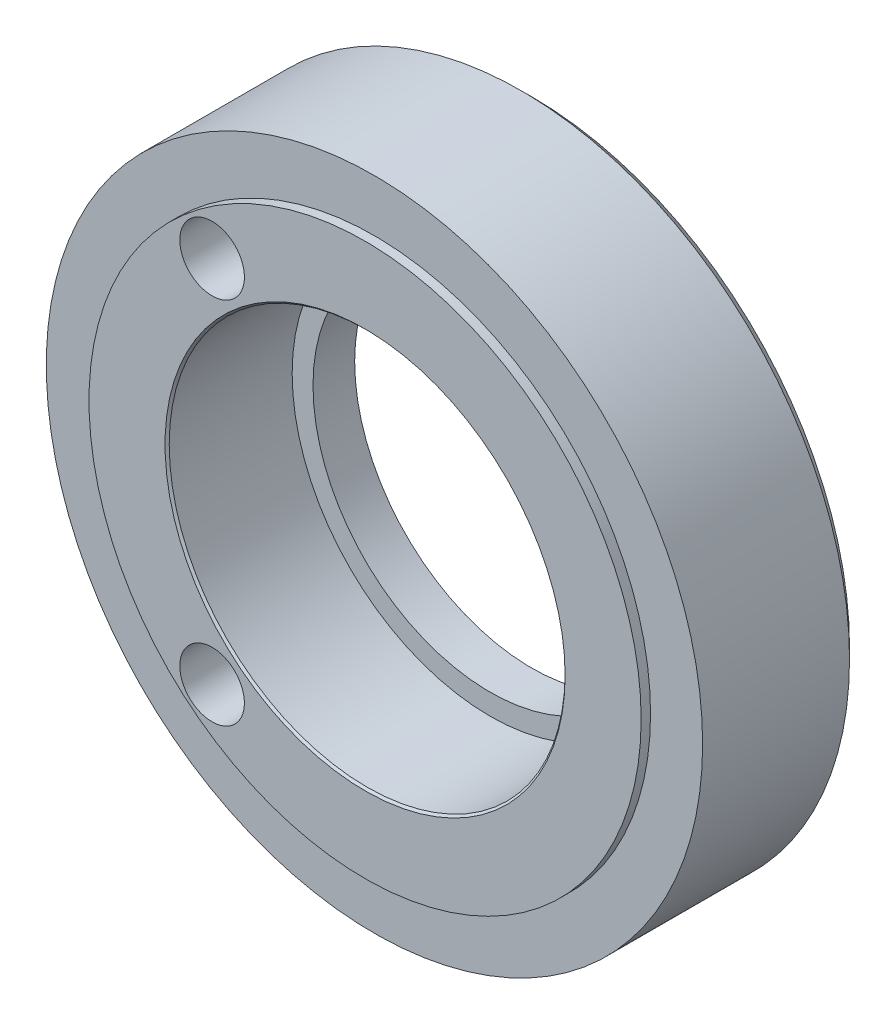
from build123d import *

# Parameters (mm, degrees)
SKETCH1_R                  = 15.75
SKETCH1_R_2                = 9.5
BOSS_EXTRUDE1_DEPTH        = 4
SKETCH3_R                  = 10.639095477
SKETCH3_R_2                = 8.5
BOSS_EXTRUDE2_DEPTH        = 2
F_3_1_3_1_DIAMETER_HOLE1_D = 3.1
SKETCH7_R                  = 18.245705154
SKETCH7_R_2                = 13.25
CUT_EXTRUDE1_DEPTH         = 0.45
CHAMFER1_SIZE              = 0.5
CHAMFER2_SIZE              = 0.1


with BuildPart() as part:
    # Sketch1 → Boss-Extrude1 (new, symmetric)
    with BuildSketch(Plane.XY):
        Circle(SKETCH1_R)
        Circle(SKETCH1_R_2, mode=Mode.SUBTRACT)
    extrude(amount=BOSS_EXTRUDE1_DEPTH, both=True)

    # Sketch3 → Boss-Extrude2 (add)
    with BuildSketch(Plane(origin=(0, 0, -4), x_dir=(-1, 0, 0), z_dir=(0, 0, -1))):
        Circle(SKETCH3_R)
        Circle(SKETCH3_R_2, mode=Mode.SUBTRACT)
    extrude(amount=-BOSS_EXTRUDE2_DEPTH)

    # Ø3.1 (3.1) Diameter Hole1 (through all)
    with Locations(Plane(origin=(0, 0, -4), x_dir=(-1, 0, 0), z_dir=(0, 0, -1))):
        with Locations((7.341654592, 8.851559628)):
            f_3_1_3_1_diameter_hole1 = Hole(F_3_1_3_1_DIAMETER_HOLE1_D / 2)

    # Mirror1: Ø3.1 (3.1) Diameter Hole1 across plane
    add(f_3_1_3_1_diameter_hole1.mirror(Plane.ZX), mode=Mode.SUBTRACT)

    # Sketch7 → Cut-Extrude1 (cut)
    with BuildSketch(Plane.XY.offset(4)):
        Circle(SKETCH7_R)
        Circle(SKETCH7_R_2, mode=Mode.SUBTRACT)
    extrude(amount=-CUT_EXTRUDE1_DEPTH, mode=Mode.SUBTRACT)

    # Chamfer1
    chamfer1_edges = [part.edges().sort_by_distance(p)[0] for p in [
        (-15.75, 0, -4),
    ]]
    chamfer(chamfer1_edges, length=CHAMFER1_SIZE)

    # Chamfer2
    chamfer2_edges = [part.edges().sort_by_distance(p)[0] for p in [
        (-9.5, 0, 4),
    ]]
    chamfer(chamfer2_edges, length=CHAMFER2_SIZE)


solid = part.part
